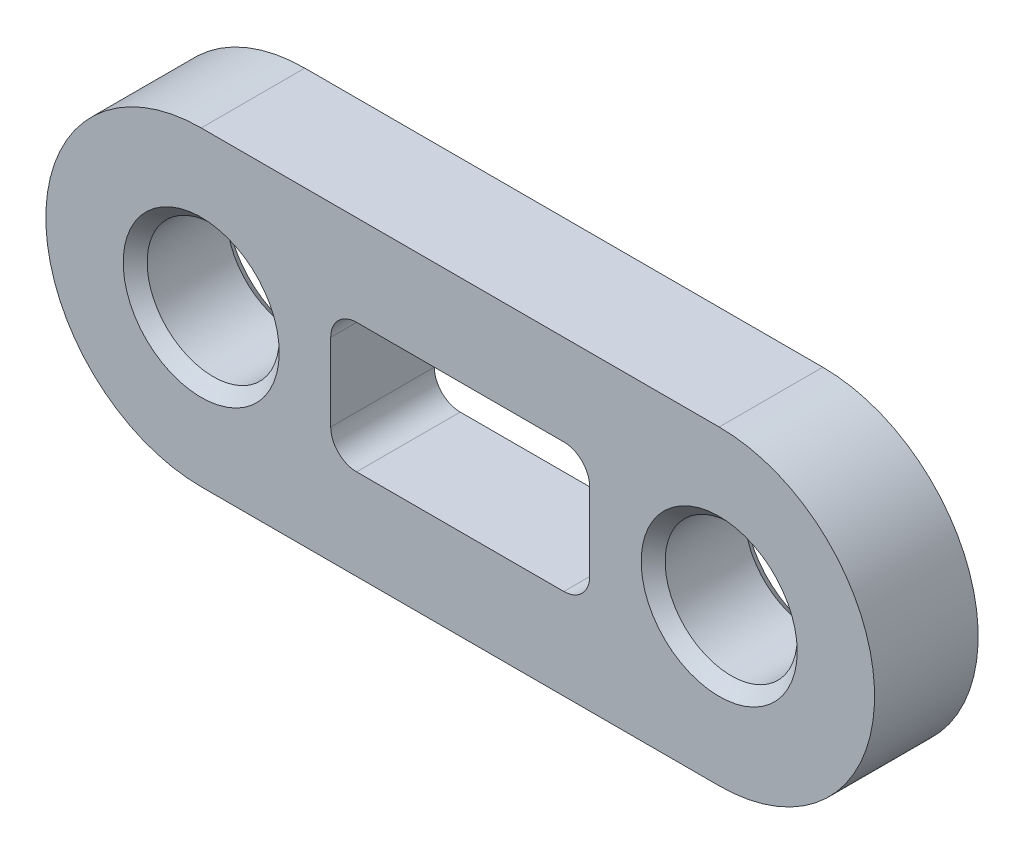
from build123d import *

# Parameters (mm, degrees)
BOSS_EXTRUDE1_DEPTH = 4


with BuildPart() as part:
    # Sketch1 → Boss-Extrude1 (new, symmetric)
    with BuildSketch(Plane.XY):
        with BuildLine():
            Line((0, 12), (40, 12))
            ThreePointArc((40, 12), (52, 0), (40, -12))
            Line((40, -12), (0, -12))
            ThreePointArc((0, -12), (-12, 0), (0, 12))
        make_face()
        with BuildLine():
            Line((12, -5), (28, -5))
            ThreePointArc((28, -5), (29.414213562, -4.414213562), (30, -3))
            Line((30, -3), (30, 3))
            ThreePointArc((30, 3), (29.414213562, 4.414213562), (28, 5))
            Line((28, 5), (12, 5))
            ThreePointArc((12, 5), (10.585786438, 4.414213562), (10, 3))
            Line((10, 3), (10, -3))
            ThreePointArc((10, -3), (10.585786438, -4.414213562), (12, -5))
        make_face(mode=Mode.SUBTRACT)
    extrude(amount=BOSS_EXTRUDE1_DEPTH, both=True)

    # Sketch2 → M12 Tapped Hole1 (revolve, cut)
    with BuildSketch(Plane(origin=(0, 0, 4), x_dir=(0, -1, 0), z_dir=(1, 0, 0))):
        Polygon((0, 0), (0, 32.75), (5.1, 29.685610843), (5.1, 0.925), (6.025, 0), align=None)
    m12_tapped_hole1 = revolve(axis=Axis((0, 0, 10.35), (0, 0, -1)), mode=Mode.SUBTRACT)

    # Mirror1: M12 Tapped Hole1 across plane
    add(m12_tapped_hole1.mirror(Plane.XY), mode=Mode.SUBTRACT)

    # Mirror2: M12 Tapped Hole1 across plane
    add(m12_tapped_hole1.mirror(Plane(origin=(20, 0, 0), x_dir=(0, 0, 1), z_dir=(1, 0, 0))), mode=Mode.SUBTRACT)

    # Mirror2 copy 1 sketch → Mirror2 copy 1 (revolve, cut)
    with BuildSketch(Plane(origin=(40, 0, -4), x_dir=(0, -1, 0), z_dir=(-1, 0, 0))):
        Polygon((0, 0), (0, 32.75), (5.1, 29.685610843), (5.1, 0.925), (6.025, 0), align=None)
    revolve(axis=Axis((40, 0, -10.35), (0, 0, 1)), mode=Mode.SUBTRACT)


solid = part.part
